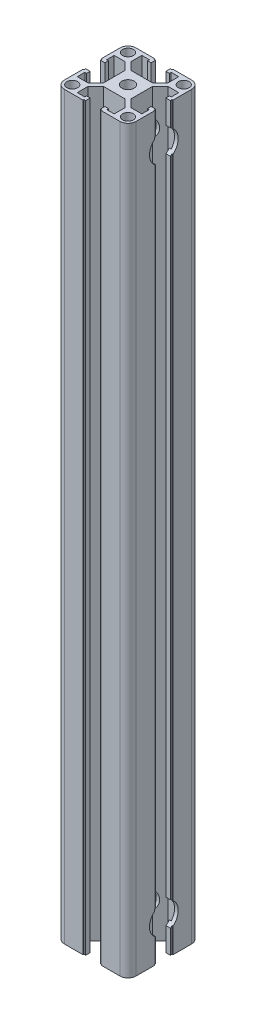
SolidWorks part; units mm, degrees
ref_plane "主视基准图" through (0, 0, 0) normal (0, 0, 1) x (1, 0, 0)
ref_plane "上视基准图" through (0, 0, 0) normal (0, 1, 0) x (1, 0, 0)
ref_plane "右视基准图" through (0, 0, 0) normal (1, 0, 0) x (0, 0, -1)
sketch "草图1" plane through (0, 0, 0) normal (0, 0, 1) x (1, 0, 0)
  line L0 (0, 0) -> (0, 413)
  dimension "D1" = 413
other "结构构件1"
ref_plane "基准面1" through (0, 0, 0) normal (0, 1, 0) x (-1, 0, 0)
sketch "Sketch16" plane through (0, 0, 0) normal (0, 1, 0) x (-1, 0, 0)
  line L0 (-5.1, 20) -> (-5.1, 19.5)
  line L1 (-5.1, 19.5) -> (-4.1, 19.5)
  line L2 (-4.1, 19.5) -> (-4.1, 17)
  line L3 (-6.1, 18) -> (-10.3, 18)
  line L4 (-15.5, -20) -> (-5.1, -20)
  line L5 (-20, -15.5) -> (-20, -5.1)
  line L6 (15.5, 20) -> (5.1, 20)
  line L7 (20, 15.5) -> (20, 5.1)
  line L8 (0, 14.8756) -> (0, 0) construction
  line L9 (0, 0) -> (14.1675, 0) construction
  line L10 (-10.3, 18) -> (-10.3, 12)
  line L11 (-10.3, 12) -> (-6, 7.7)
  line L12 (-6, 7.7) -> (6, 7.7)
  line L13 (10.3, 12) -> (6, 7.7)
  line L14 (10.3, 18) -> (10.3, 12)
  line L15 (6.1, 18) -> (10.3, 18)
  line L16 (4.1, 19.5) -> (4.1, 17)
  line L17 (5.1, 19.5) -> (4.1, 19.5)
  line L18 (5.1, 20) -> (5.1, 19.5)
  line L19 (-5.1, 20) -> (-15.5, 20)
  line L20 (20, 5.1) -> (19.5, 5.1)
  line L21 (0, 0) -> (-15.5563, 15.5563) construction
  line L22 (0, 0) -> (-15.5563, -15.5563) construction
  line L25 (19.5, 5.1) -> (19.5, 4.1)
  line L26 (19.5, 4.1) -> (17, 4.1)
  line L27 (17, 6.1) -> (17, 4.1)
  line L28 (18, 6.1) -> (17, 6.1)
  line L29 (18, 6.1) -> (18, 10.3)
  line L30 (18, 10.3) -> (12, 10.3)
  line L31 (12, 10.3) -> (7.7, 6)
  line L32 (7.7, 6) -> (7.7, -6)
  line L33 (12, -10.3) -> (7.7, -6)
  line L34 (18, -10.3) -> (12, -10.3)
  line L35 (18, -6.1) -> (18, -10.3)
  line L36 (18, -6.1) -> (17, -6.1)
  line L37 (17, -4.1) -> (17, -6.1)
  line L38 (19.5, -4.1) -> (17, -4.1)
  line L39 (19.5, -5.1) -> (19.5, -4.1)
  line L40 (20, -5.1) -> (19.5, -5.1)
  line L41 (5.1, -20) -> (5.1, -19.5)
  line L42 (5.1, -19.5) -> (4.1, -19.5)
  line L43 (4.1, -19.5) -> (4.1, -17)
  line L44 (6.1, -17) -> (4.1, -17)
  line L45 (6.1, -18) -> (6.1, -17)
  line L46 (6.1, -18) -> (10.3, -18)
  line L47 (10.3, -18) -> (10.3, -12)
  line L48 (10.3, -12) -> (6, -7.7)
  line L49 (6, -7.7) -> (-6, -7.7)
  line L50 (-10.3, -12) -> (-6, -7.7)
  line L51 (-10.3, -18) -> (-10.3, -12)
  line L52 (-6.1, -18) -> (-10.3, -18)
  line L53 (-6.1, -18) -> (-6.1, -17)
  line L54 (-4.1, -17) -> (-6.1, -17)
  line L55 (-4.1, -19.5) -> (-4.1, -17)
  line L56 (-5.1, -19.5) -> (-4.1, -19.5)
  line L57 (-5.1, -20) -> (-5.1, -19.5)
  line L58 (-20, -5.1) -> (-19.5, -5.1)
  line L59 (5.1, -20) -> (15.5, -20)
  line L60 (-20, 5.1) -> (-20, 15.5)
  line L61 (-19.5, -5.1) -> (-19.5, -4.1)
  line L62 (-6.1, 18) -> (-6.1, 17)
  line L63 (-6.1, 17) -> (-4.1, 17)
  line L64 (6.1, 18) -> (6.1, 17)
  line L65 (4.1, 17) -> (6.1, 17)
  line L66 (-19.5, -4.1) -> (-17, -4.1)
  line L71 (-17, -6.1) -> (-17, -4.1)
  line L72 (-18, -6.1) -> (-17, -6.1)
  line L73 (-18, -6.1) -> (-18, -10.3)
  line L74 (-18, -10.3) -> (-12, -10.3)
  line L75 (-12, -10.3) -> (-7.7, -6)
  line L76 (-7.7, -6) -> (-7.7, 6)
  line L77 (-12, 10.3) -> (-7.7, 6)
  line L78 (-18, 10.3) -> (-12, 10.3)
  line L79 (-18, 6.1) -> (-18, 10.3)
  line L80 (-18, 6.1) -> (-17, 6.1)
  line L81 (-17, 4.1) -> (-17, 6.1)
  line L82 (-19.5, 4.1) -> (-17, 4.1)
  line L83 (-19.5, 5.1) -> (-19.5, 4.1)
  line L84 (-20, 5.1) -> (-19.5, 5.1)
  line L85 (20, -5.1) -> (20, -15.5)
  circle A0 centre (0, 0) radius 3.4
  arc A1 (-20, 15.5) -> (-15.5, 20) centre (-15.5, 15.5) cw
  arc A2 (20, 15.5) -> (15.5, 20) centre (15.5, 15.5) ccw
  arc A3 (-15.5, -20) -> (-20, -15.5) centre (-15.5, -15.5) cw
  arc A4 (15.5, -20) -> (20, -15.5) centre (15.5, -15.5) ccw
  circle A5 centre (-15.5563, 15.5563) radius 3
  circle A6 centre (15.5563, 15.5563) radius 3
  circle A7 centre (15.5563, -15.5563) radius 3
  circle A8 centre (-15.5563, -15.5563) radius 3
  point P2 (0, 10)
  point P3 (0, 0)
  point P4 (0, 0)
  point P5 (-20, -20)
  point P6 (20, -20)
  point P7 (20, 20)
  point P8 (-20, 20)
  point P36 (-20, 20)
  point P39 (20, 20)
  dimension "D1" = 20.6
  dimension "D2" = 40
  dimension "D3" = 8.2
  dimension "D4" = 10.2
  dimension "D5" = 12.3
  dimension "D6" = 6.8
  dimension "D7" = 4.5
  dimension "D8" = 45
  dimension "D12" = 6
  dimension "D13" = 22
  dimension "D9" = 0.5
  dimension "D10" = 2
  dimension "D11" = 12
  dimension "D16" = 3
  dimension "D17" = 2
hole_wizard "M8 六角凹头螺钉的柱形沉头孔1" positions "草图3" profile "草图2" counterbore size "M8" standard "Iso" end condition through all
sketch "草图3" plane through (20, 0, 0) normal (1, 0, 0) x (0, 0, -1)
  line L1 (0, 413) -> (0, 0) construction
  line L2 (-15.5, 413) -> (-5.1, 413) construction
  line L3 (-15.5, 0) -> (-5.1, 0) construction
  point P0 (0, 20)
  point P2 (0, 393)
  dimension "D1" = 20
  dimension "D2" = 20
sketch "草图2" plane through (20, 20, 0) normal (0, 1, 0) x (0, 0, -1)
  line L0 (0, 0) -> (0, 40)
  line L1 (0, 40) -> (4.5, 40)
  line L3 (4.5, 40) -> (4.5, 12.3)
  line L4 (4.5, 12.3) -> (8, 12.3)
  line L5 (8, 12.3) -> (8, 0)
  line L7 (8, 0) -> (0, 0)
  line L11 (0, -6.35) -> (0, 107.95) construction
  dimension "通孔孔直径" = 9
  dimension "通孔孔深度" = 40
  dimension "柱形沉头孔直径" = 16
  dimension "柱形沉头孔深度" = 12.3
